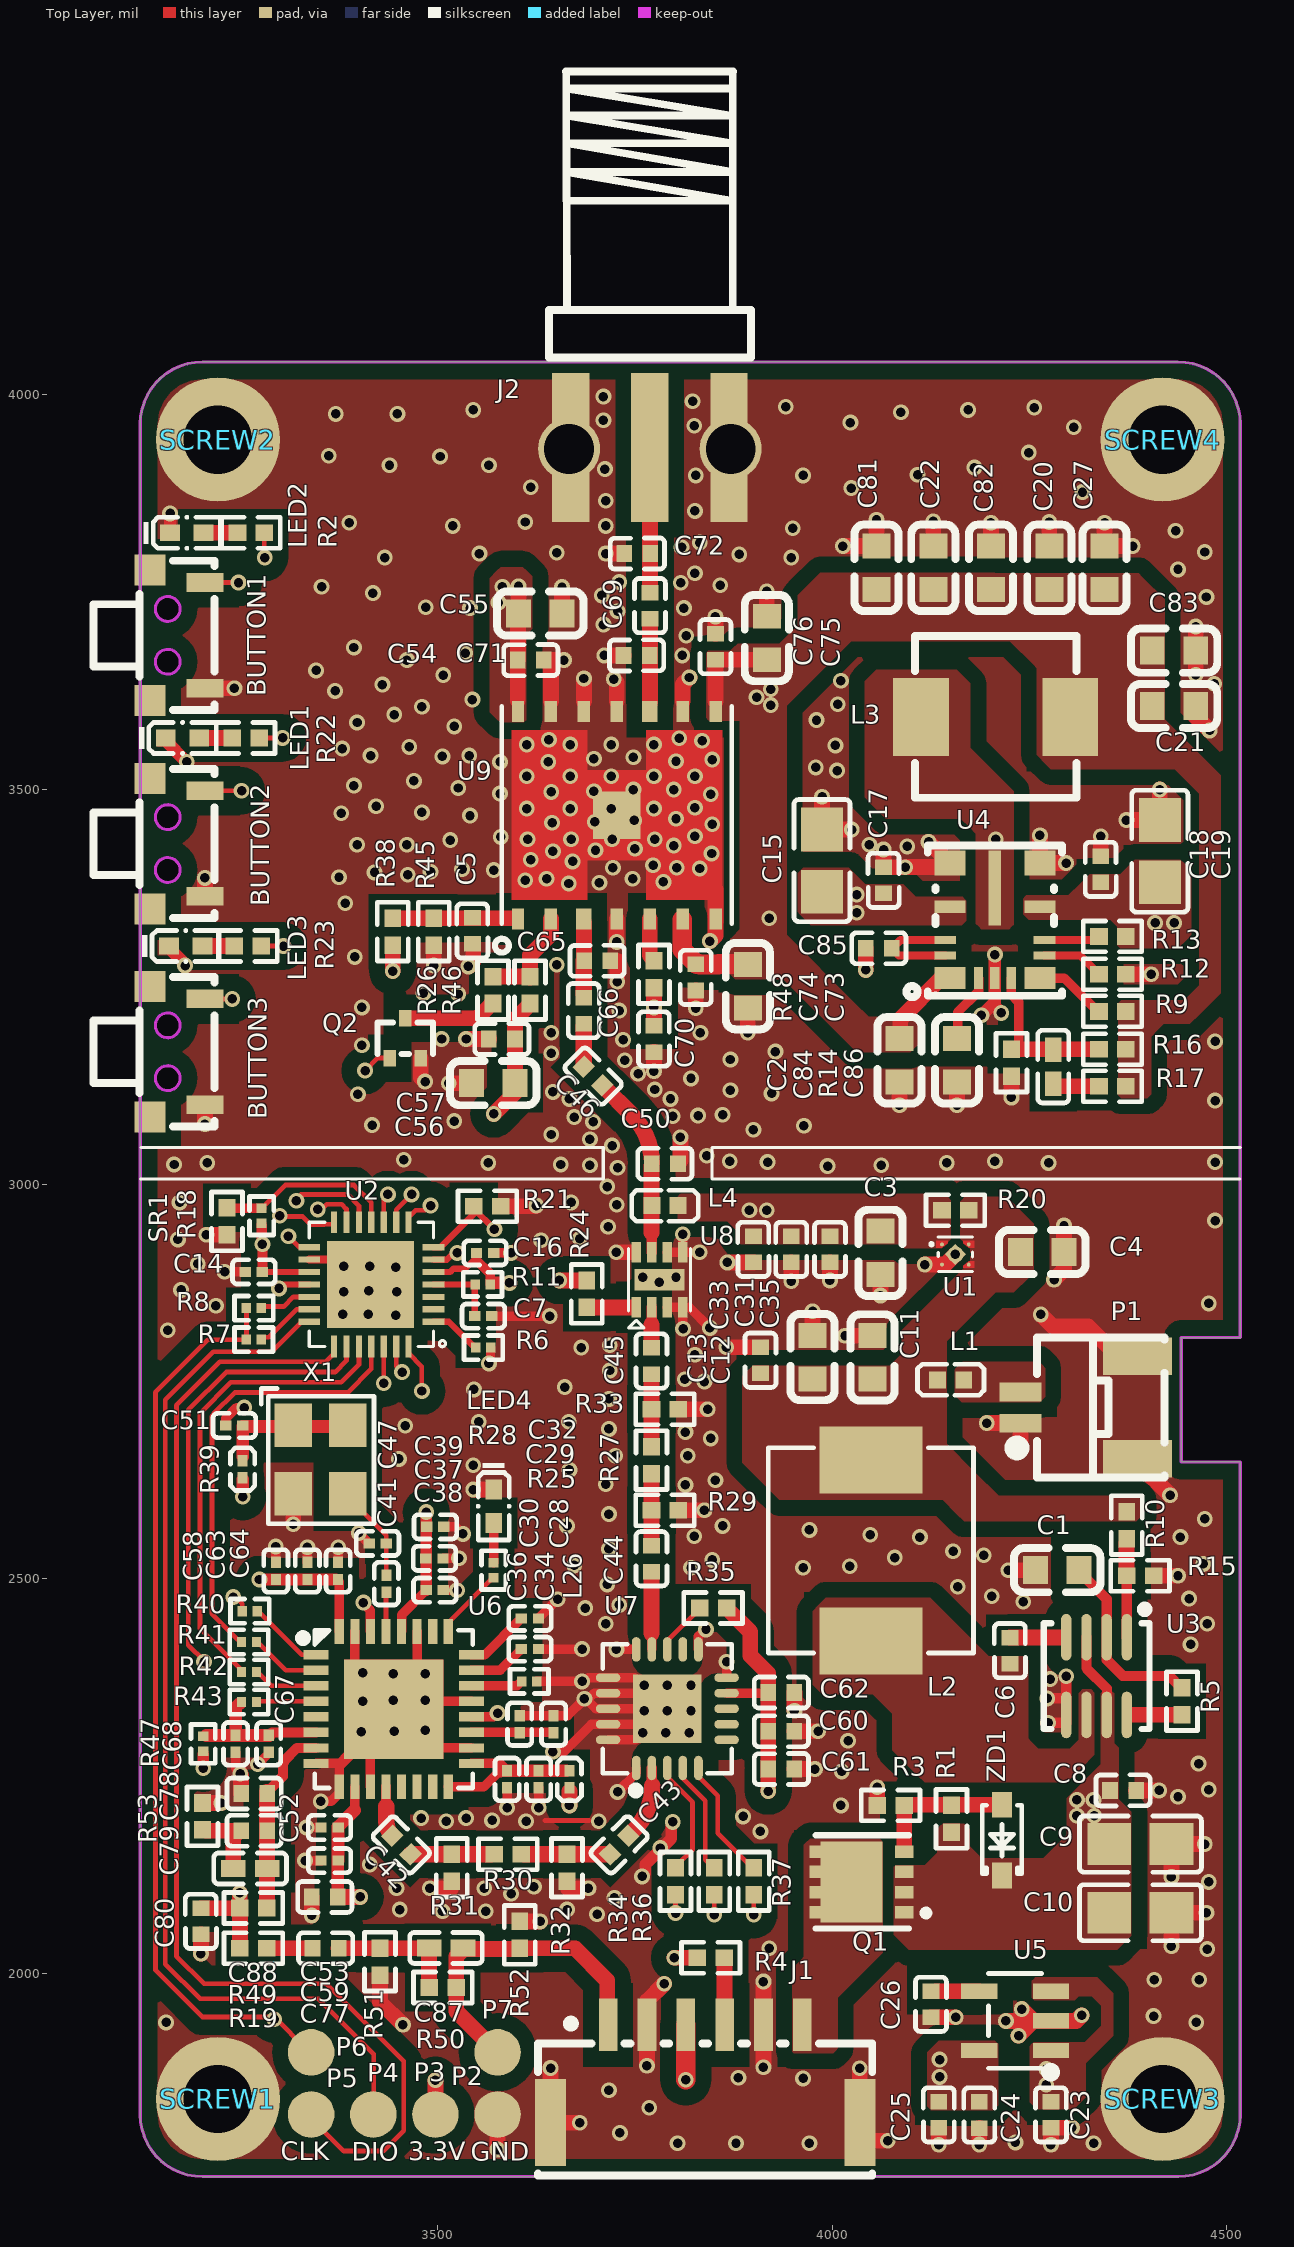
[diagram p0: Top Layer view]
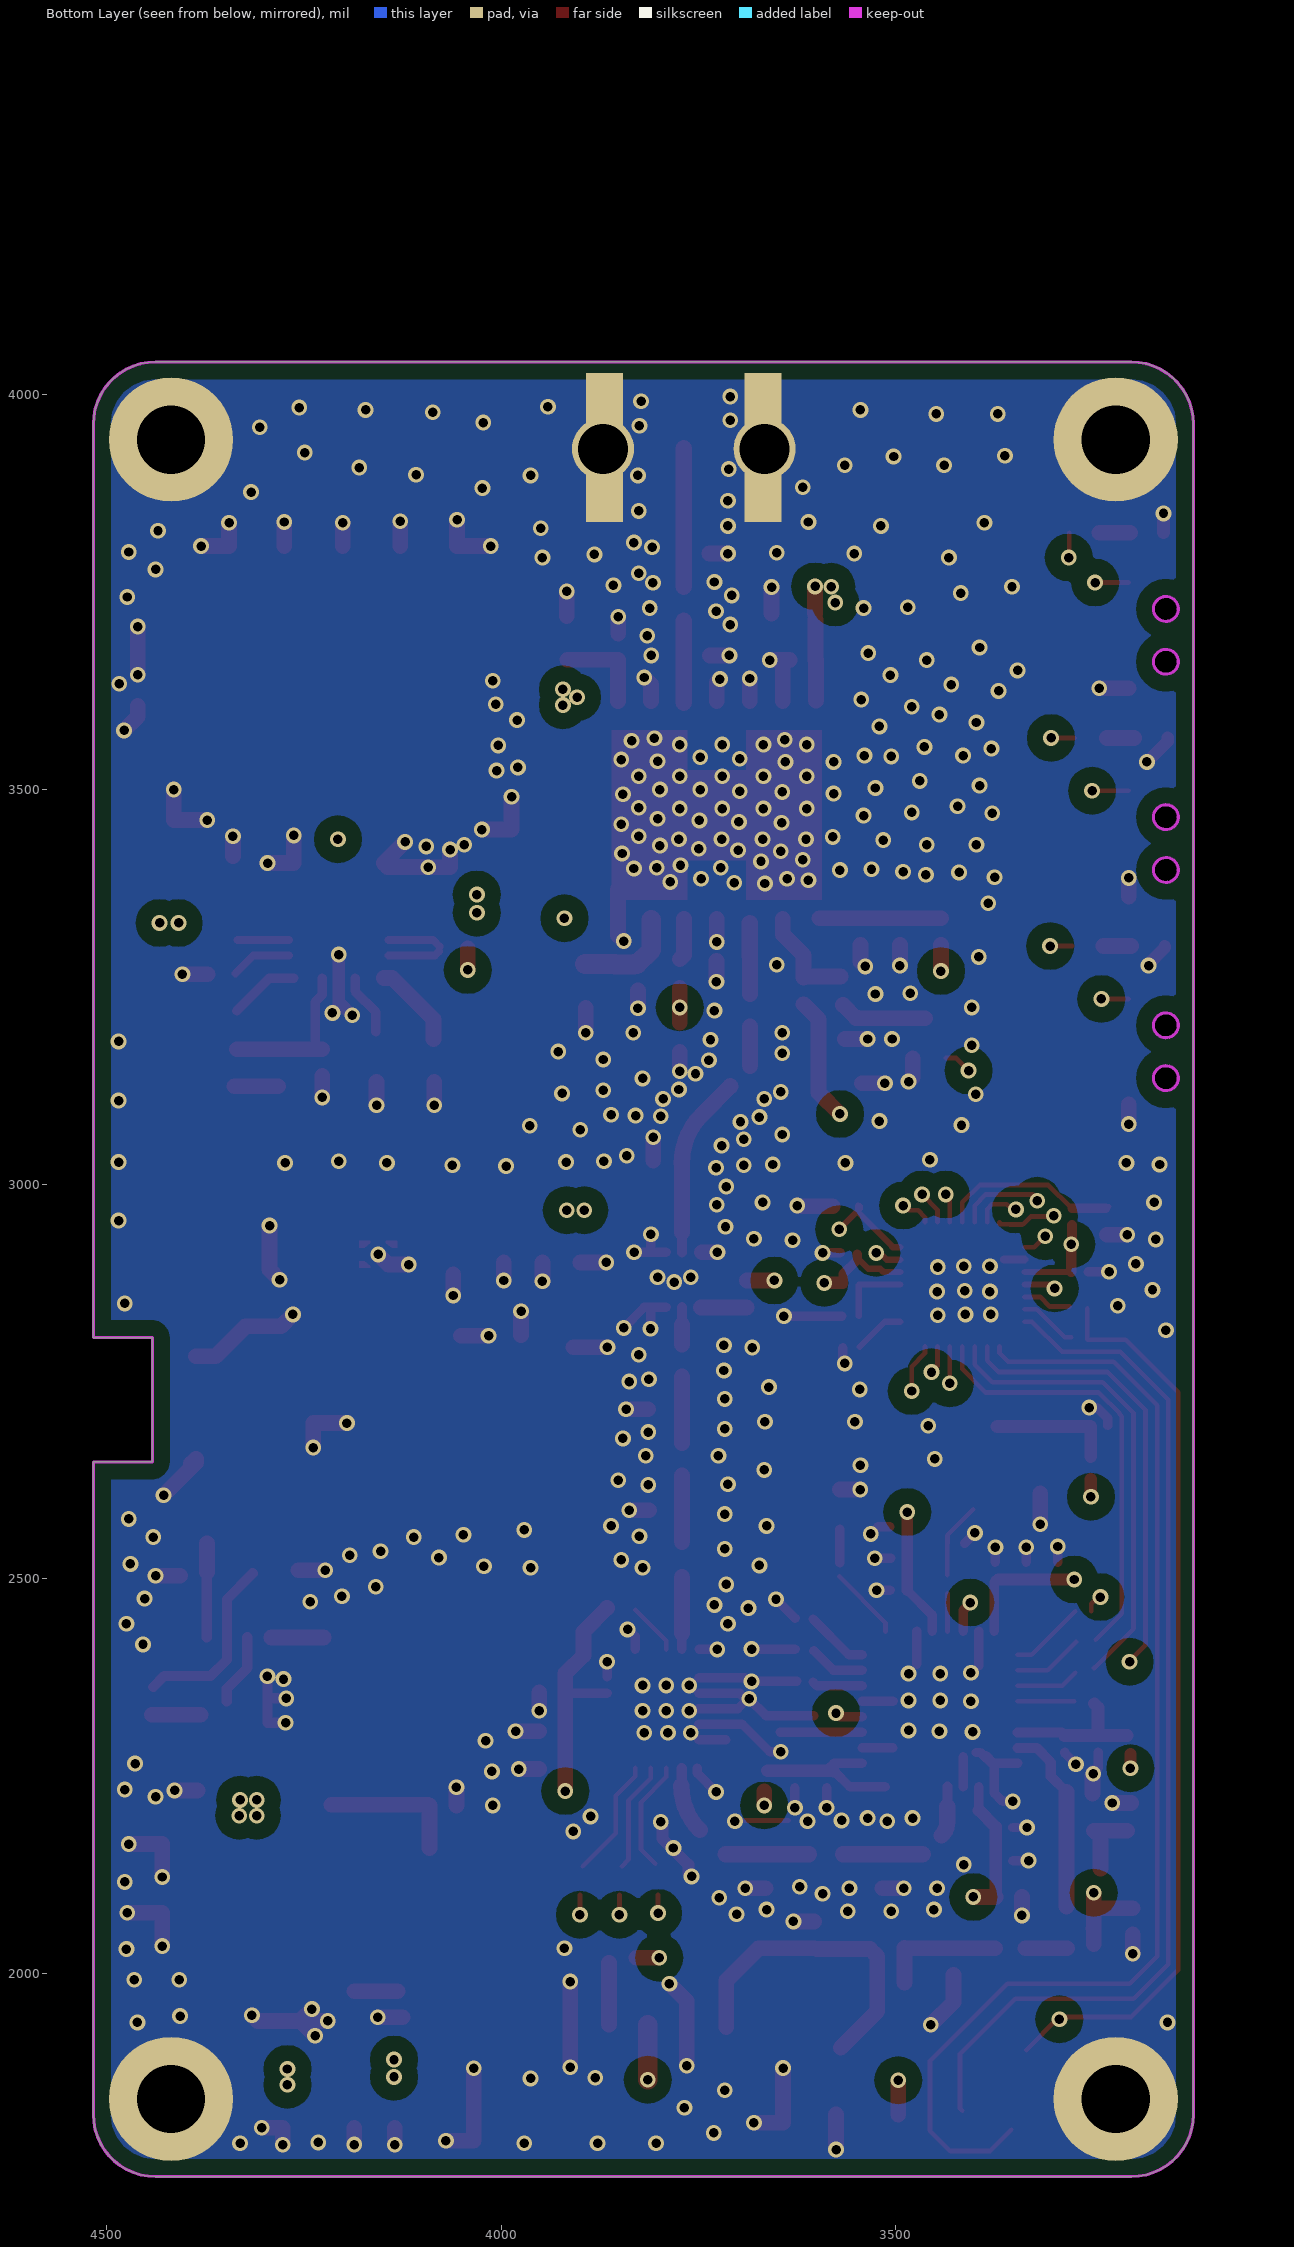
[diagram p1: Bottom Layer view, seen from below]
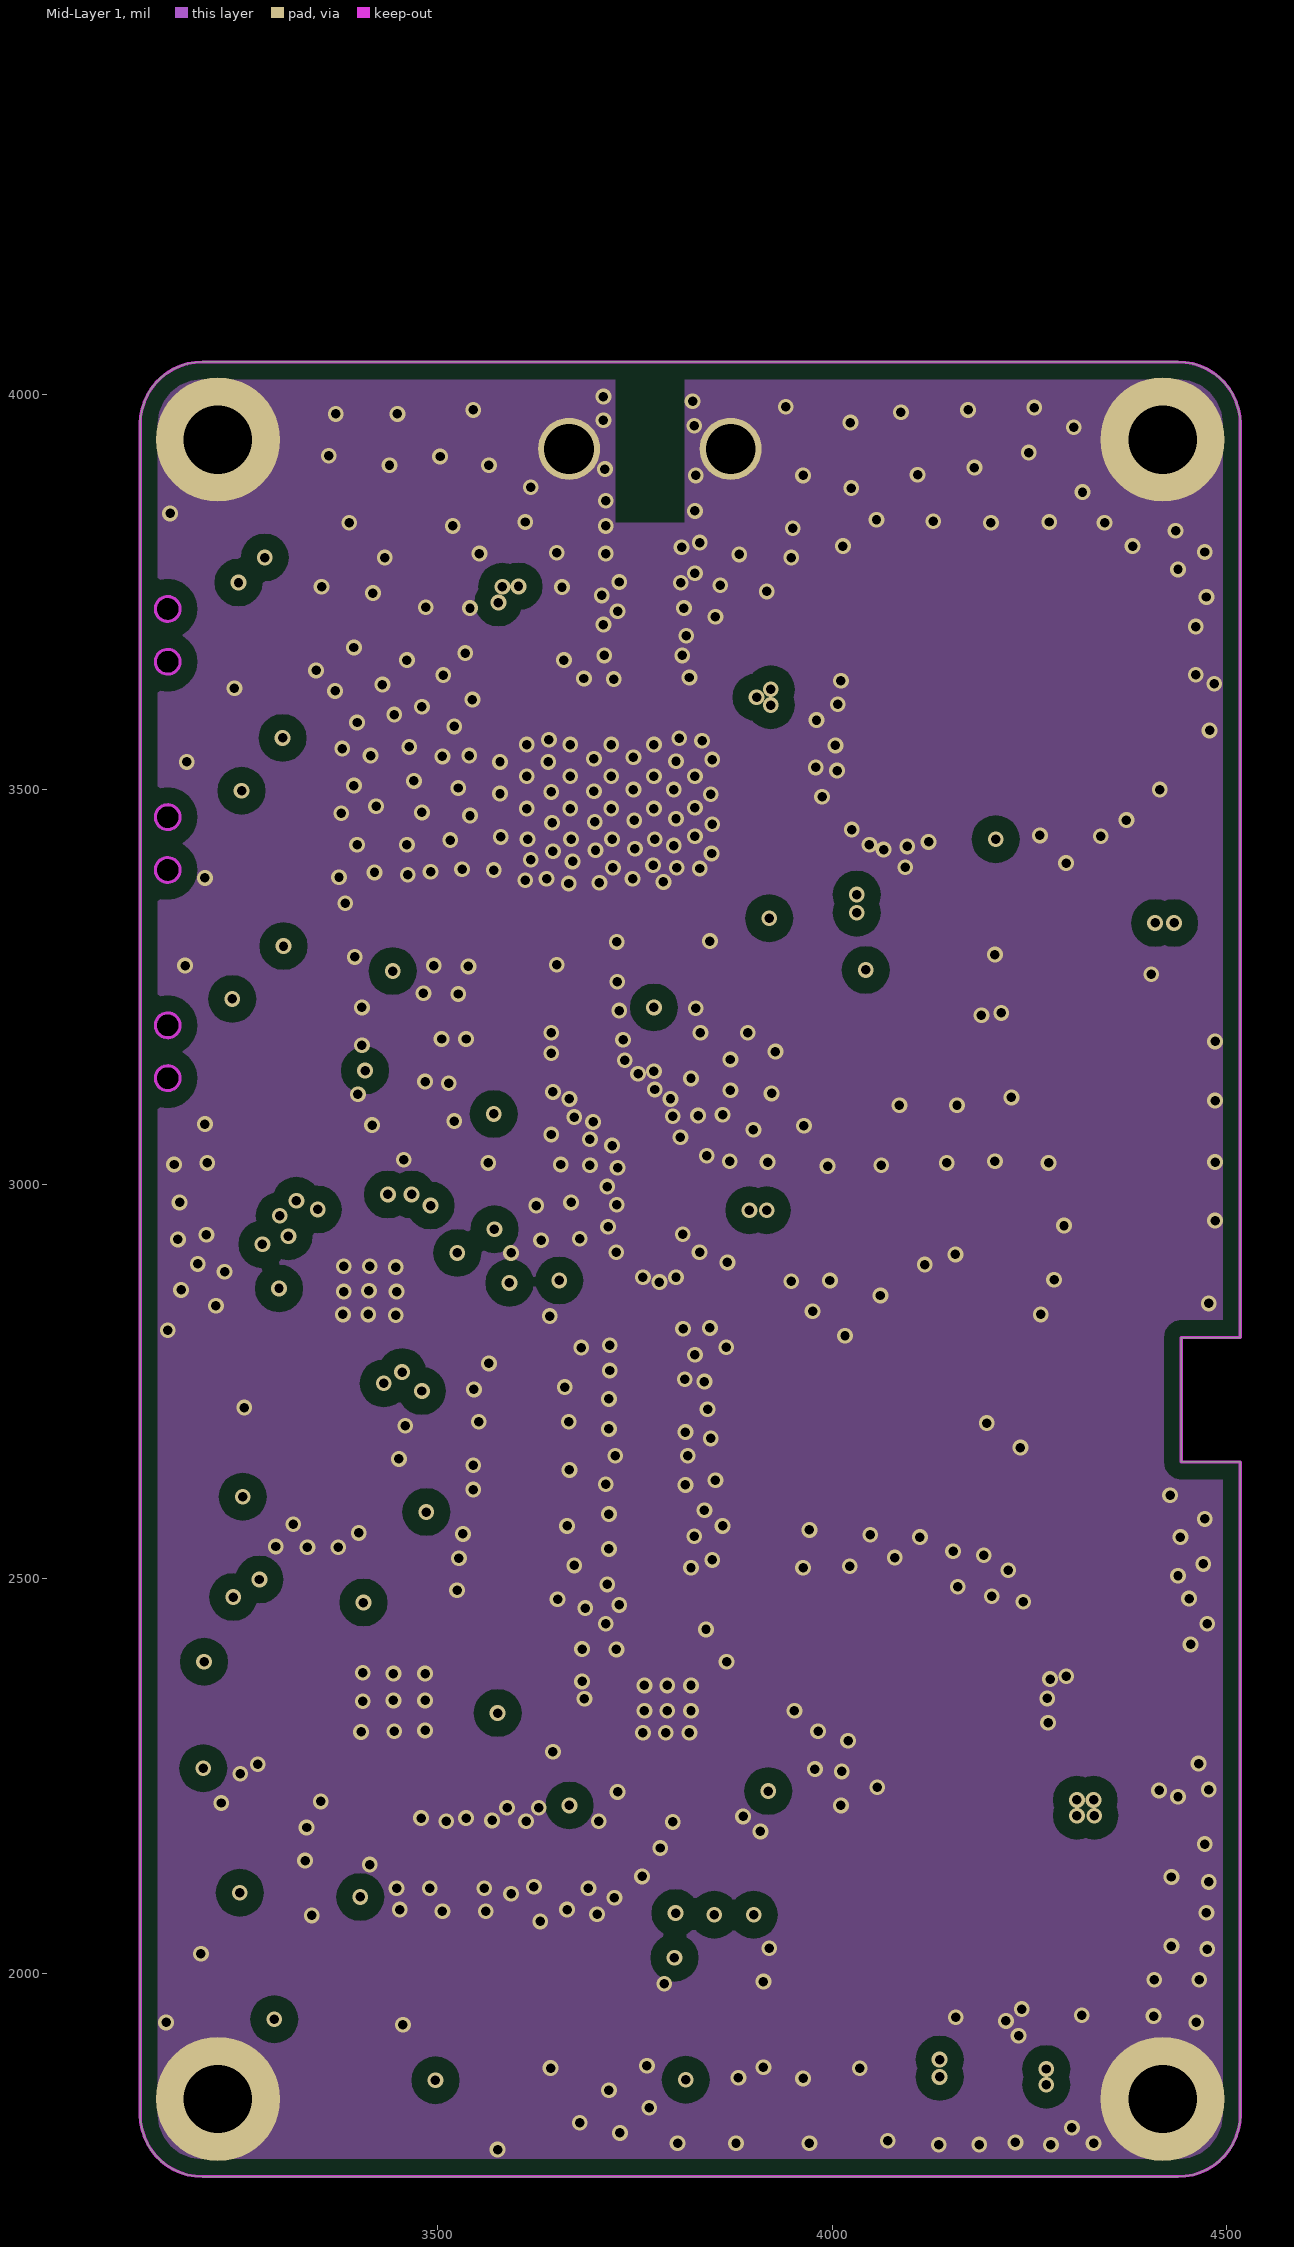
[diagram p2: Mid-Layer 1]
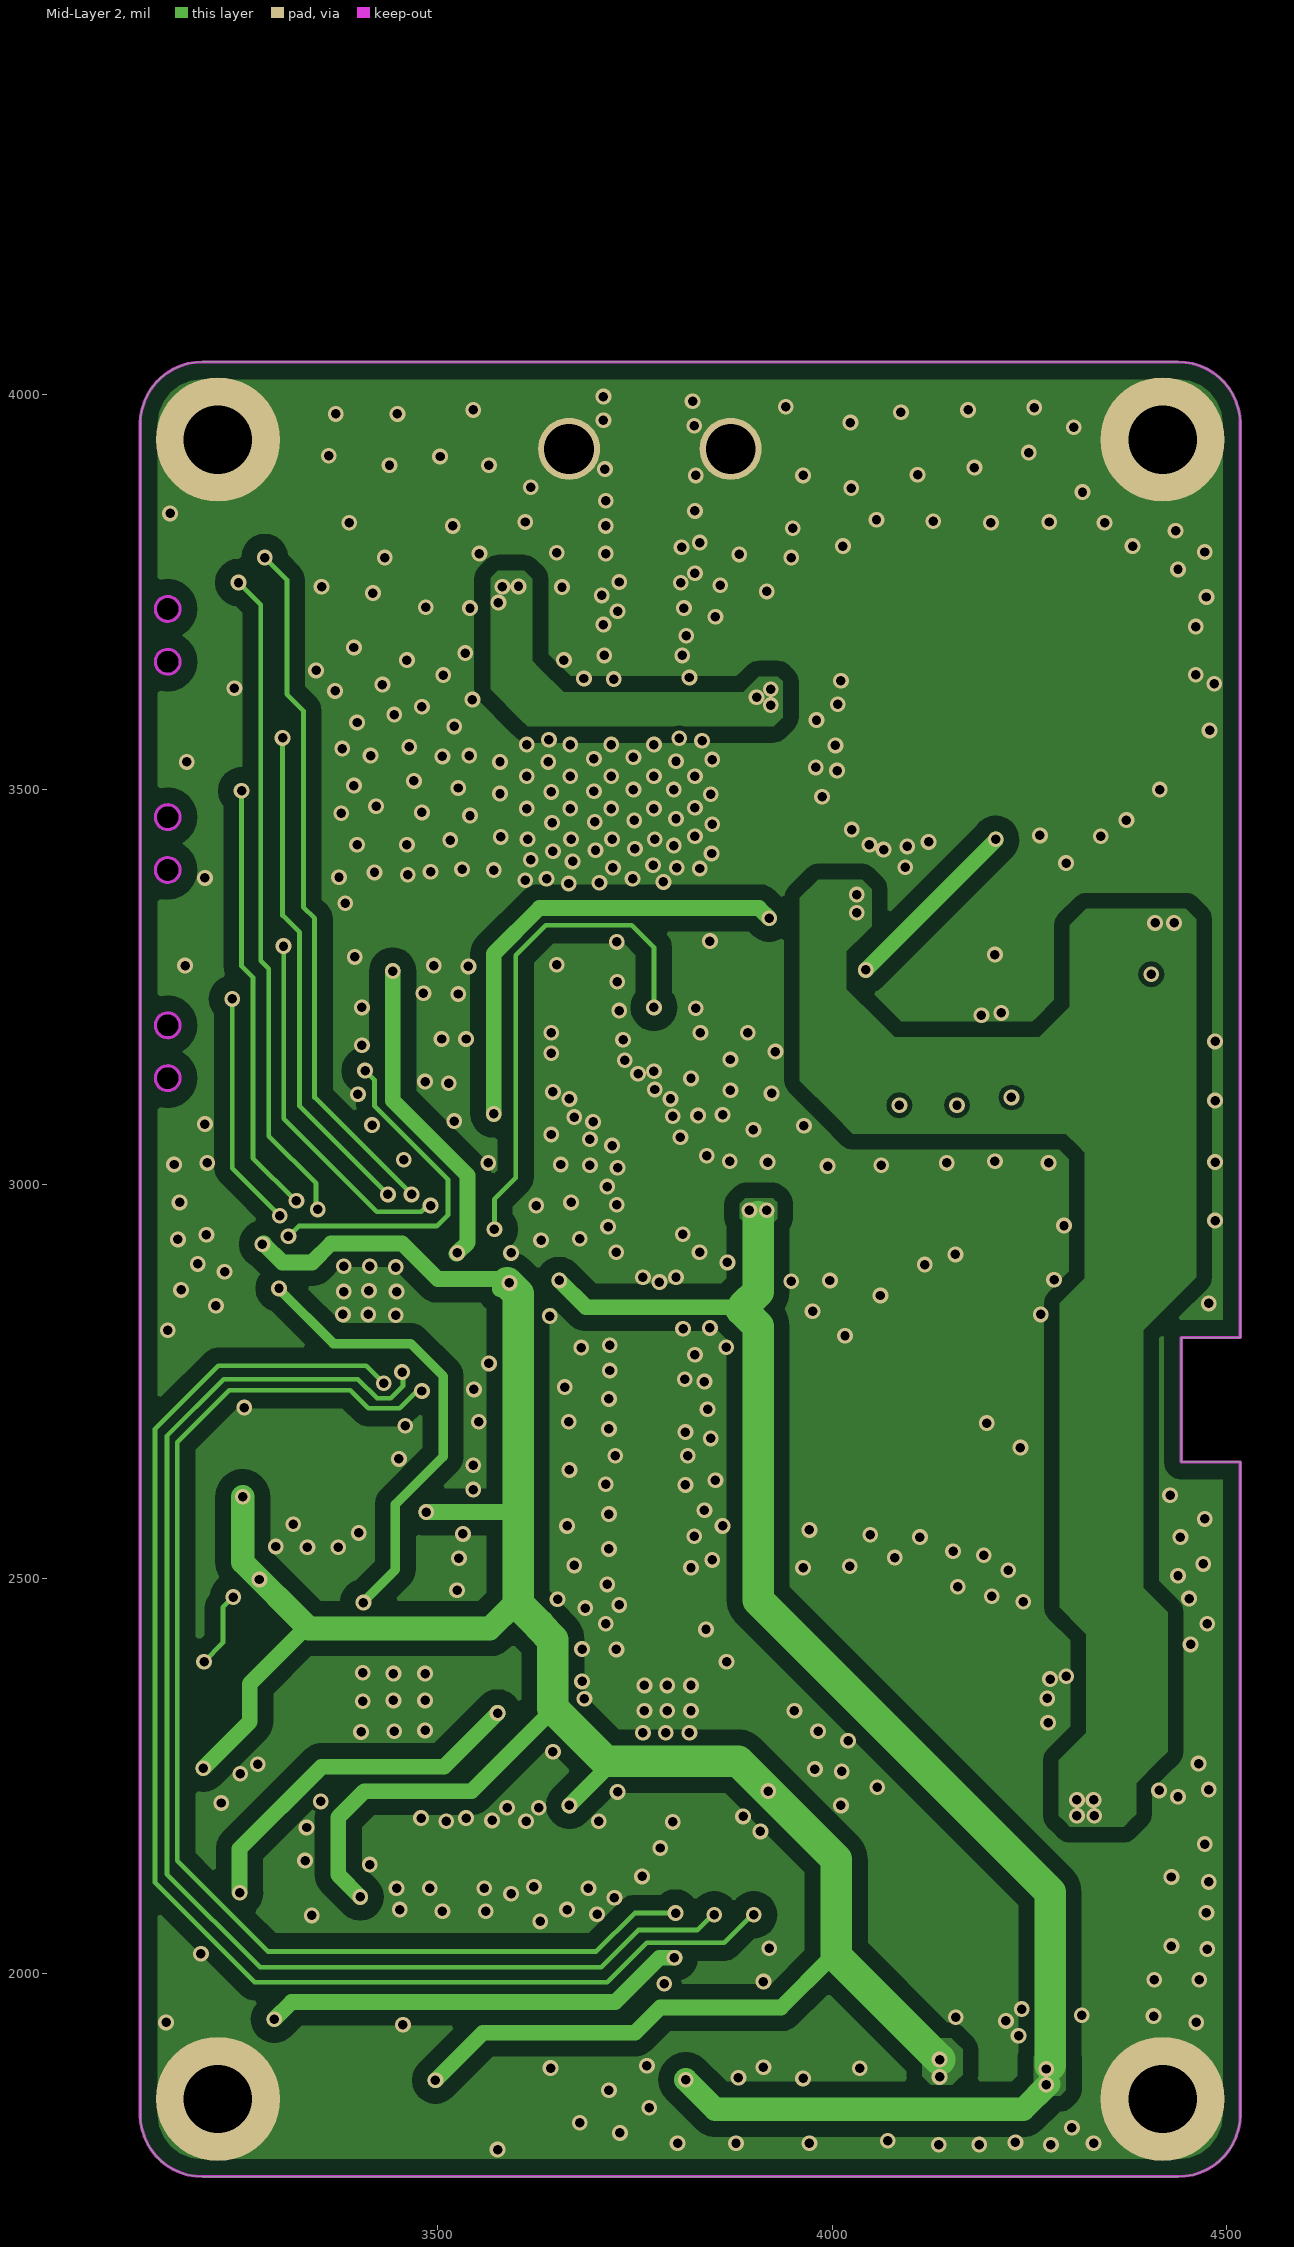
[diagram p3: Mid-Layer 2]
# Altium PCB MISC62792.PcbDoc (part 1 of 2)
Units mil, origin at the board's own origin, x right, y up, seen from the top; angles counter-clockwise.
Board outline 1393.7 x 2299.21 mil, 4 copper layers (Top Layer, Mid-Layer 1, Mid-Layer 2, Bottom Layer); 176 components, 94 nets, 498 pads, 570 vias.

## Layer stack, top to bottom (the 12.6 mil dielectric is the usual default, probably not edited)
Top Layer: signal copper 1.4
Dielectric: core 12.6, FR-4, Dk 4.8
Mid-Layer 1: signal copper 1.4
Dielectric: prepreg 12.6, FR-4, Dk 4.8
Mid-Layer 2: signal copper 1.4
Dielectric: core 12.6, FR-4, Dk 4.8
Bottom Layer: signal copper 1.4

## Board outline
3123.19,1821.38 ccw(c3201.93,1821.38) 3201.93,1742.64 4438.15,1742.64 ccw(c4438.15,1821.38) 4516.89,1821.38 4516.89,2648.15 4442.09,2648.15 4442.09,2805.63 4516.89,2805.63 4516.89,3963.11 ccw(c4438.15,3963.11) 4438.15,4041.85 3201.93,4041.85 ccw(c3201.93,3963.11) 3123.19,3963.11

## Design rules (kind name [scope] priority, off if disabled: settings)
Clearance Clearance_5 [INPOLYGON] p1: gap=6
Clearance [All] p2: gap=6
DiffPairsRouting [All] p1: maxlimit=6 minlimit=6 mostfreqgap=6 maxuncoupledlength=500
HoleSize [All] p1: absolutevalues=TRUE maxlimit=500 minlimit=1 maxpercent=80.000 minpercent=20.000
HoleToHoleClearance [All] p1: gap=0 allowstackedmicrovias=TRUE
MinimumSolderMaskSliver [All] p1: minsoldermaskwidth=0
PlaneClearance [All] p1: clearance=6
PlaneConnect [All] p1: planeconnectstyle=Direct reliefexpansion=20 reliefentries=4 reliefconductorwidth=10 reliefairgap=10
PolygonConnect [All] p1: connectstyle=Direct reliefconductorwidth=10 reliefentries=4 polygonreliefangle="90 Angle"
RoutingVias [All] p1: holewidth=12 width=20 viastyle="Through Hole" minholewidth=12 minwidth=20 maxholewidth=12 maxwidth=20
SilkToSilkClearance [All] p1: silktosilkclearance=0
SilkscreenOverComponentPads [All] p1: minsilkscreentomaskgap=0
SolderMaskExpansion [All] p1: expansion=4
Width [All] p1: maxlimit=100 minlimit=6 preferedwidth=6
20 further rules are at their usual default settings.

## Components (designator, comment, footprint, x,y, rotation, side; value= is the part's Value field where it differs from the comment)
BUTTON1 "TS24CA250GF013" SW-SMD_L4.7-W3.5-P3.35-EH 3170.43,3695.39 r0 top
BUTTON2 "TS24CA250GF013" SW-SMD_L4.7-W3.5-P3.35-EH 3170.43,3431.61 r0 top
BUTTON3 "TS24CA250GF013" SW-SMD_L4.7-W3.5-P3.35-EH 3170.43,3167.83 r0 top
C1 "1uf" C0603 4285,2511 r180 top
C2 "1uf" C0603 4085,3157 r270 top
C3 "1uF" C0603 4061,2913 r270 top
C4 "1uF" C0603 4266,2914 r0 top
C5 "0.1uF" C0402#1 3544,3321 r90 top
C6 "0.1uF" C0402#1 4225,2409 r270 top
C7 "100nf" C0201 3558,2833 r180 top
C8 "100nf" C0402#1 4368.37,2232 r0 top
C9 "10uF" C0805 4390.37,2164 r0 top
C10 "10uF" C0805 4390.37,2077 r0 top
C11 "22uF" C0603 4051,2780.56 r90 top
C12 "22uF" C0603 3975,2781 r90 top
C13 "100nf" C0402#1 3909,2777 r90 top
C14 "100nf" C0201 3267.2,2889 r180 top
C15 "10uF" C0805 3987,3410 r90 top
C16 "100nf" C0201 3560,2913 r0 top
C17 "100nf" C0402#1 4065,3385 r90 top
C18 "100nf" C0402#1 4340,3399 r90 top
C19 "10uF" C0805 4415,3422 r90 top
C20 "22uF" C0603 4275,3781 r90 top
C21 "22uF" C0603 4433,3606 r0 top
C22 "22uF" C0603 4128,3781 r90 top
C23 "1uF" C0402#1 4277,1821 r270 top
C24 "1uF" C0402#1 4186.33,1820.72 r270 top
C25 "100nf" C0402#1 4135,1821 r270 top
C26 "3.3nf" C0402#1 4125,1961 r270 top
C27 "22uF" C0603 4345,3781 r90 top
C28 "0.1uF" C0201 3647,2316 r270 top
C29 "0.1uF" C0201 3617,2411 r0 top
C30 "1NF" C0201 3604,2316 r90 top
C31 "1UF" C0402#1 3948,2917.46 r90 top
C32 "1NF" C0201 3617,2450 r180 top
C33 "100nf" C0402#1 3900,2917.46 r90 top
C34 "0.1uF" C0201 3628,2246 r90 top
C35 "10PF   50V" C0402#1 3997,2917.46 r270 top
C36 "1NF" C0201 3588,2246 r270 top
C37 "0.1uF" C0201 3496,2526 r180 top
C38 "1NF" C0201 3496.46,2485.62 r0 top
C39 "0.1uF" C0201 3497,2566 r180 top
C41 "1NF" C0201 3435,2494 r90 top
C42 "10PF" C0402#1 3454,2163 r315 top
C43 "10PF" C0402#1 3730,2163 r45 top
C44 "10PF" C0402#1 3771,2525.46 r90 top
C45 "10PF" C0402#1 3771,2776 r90 top
C46 "10PF" C0402#1 3697,3137 r135 top
C47 "1NF" C0201 3424,2545 r180 top
C50 "NC" C0402#1 3788,3026 r0 top
C51 "1NF" C0201 3242.35,2694.31 r0 top
C52 "100PF" C0201 3363,2185 r180 top
C53 "0.1uF" C0201 3363,2143 r0 top
C54 "10PF" C0402#1 3618,3664 r0 top
C55 "4.7UF" C0603 3630,3723 r0 top
C56 "4.7UF" C0603 3570.46,3128 r0 top
C57 "10PF" C0402#1 3581.46,3184 r0 top
C58 "1NF" C0201 3295,2510 r270 top
C59 "10uF" C0402#1 3357,2097 r0 top
C60 "1NF" C0402#1 3935.46,2307 r180 top
C61 "100nf" C0402#1 3935.46,2259 r180 top
C62 "1UF" C0402#1 3935.46,2356 r180 top
C63 "1NF" C0201 3335,2510 r270 top
C64 "1NF" C0201 3374,2510 r90 top
C65 "NC" C0402#1 3702,3283 r0 top
C66 "10PF" C0402#1 3685,3220 r270 top
C67 "1NF" C0201 3286,2291 r270 top
C68 "0.1uF" C0201 3244,2291 r90 top
C69 "10PF" C0402#1 3769,3733 r90 top
C70 "2.2NF" C0402#1 3774,3184 r90 top
C71 "NC" C0402#1 3752,3670 r0 top
C72 "NC" C0402#1 3753,3799 r0 top
C73 "4.7uF" C0603 3893,3251 r270 top
C74 "10PF" C0402#1 3827,3262 r270 top
C75 "4.7UF" C0603 3917,3692 r90 top
C76 "10PF" C0402#1 3852,3681 r90 top
C77 "4.7UF" C0402#1 3358,2032 r180 top
C78 "4.7UF" C0402#1 3267.42,2228 r180 top
C79 "22UF" C0402#1 3267.42,2181 r0 top
C80 "2PF" C0402#1 3200,2066 r90 top
C81 "22uF" C0603 4056,3781 r90 top
C82 "22uF" C0603 4201,3781 r90 top
C83 "1uf" C0603 4433,3676 r0 top
C84 "1uf" C0603 4158,3157 r270 top
C85 "0.1uF" C0402#1 4059,3299 r180 top
C86 "22pF" C0402#2 4280,3149 r270 top
C87 "150PF" C0402#2 3510.63,2032.41 r180 top
C88 "22UF" C0402#2 3262.42,2133 r0 top
J1 "WAFER-GH1. 25-6PWB" SMD_6P-P1.25_XUNPU_WAFER-GH1.25-6PWB 3838.98,1872.99 r0 top locked
J2 "SMA-50KE-3" SMA-FP-945G 3768.86,3931.61 r90 top locked
L1 "MPZ1005S121CT000" L0402 4150,2752 r180 top
L2 "SL0624-100M" IND-SMD_L7.1-W6.6 4049,2536 r90 top
L3 "MCS0530-4R7MN2" IND-SMD_L5.2-W5.2_YSPI0530 4207,3592 r0 top
L4 "33nH" L0402 3788,2973 r0 top
L26 "BLM03PX800SN1D" L0201 3667,2246 r90 top
LED1 "LED" LED0402 3176.8,3565.47 r0 top
LED2 "LED" LED0402 3182.24,3825.31 r0 top
LED3 "LED" LED0402 3180.74,3301.69 r0 top
LED4 "LED" LED0402 3571,2592 r270 top
P1 "WAFER-SHB1.0-2PWB" SMD_2P-WAFER-SHB1.0-2PWB 4312.66,2717.05 r90 top locked
P2 "Pad" PAD 3575.94,1821.38 r0 top locked
P3 "Pad" PAD 3497.2,1821.38 r0 top locked
P4 "Pad" PAD 3418.46,1821.38 r0 top locked
P5 "Pad" PAD 3339.72,1821.38 r0 top locked
P6 "Pad" PAD 3339.72,1900.12 r0 top
P7 "Pad" PAD 3575.94,1900.12 r0 top locked
Q1 "CJAE10P06" DFN-8_L3.0-W3.0-P0.65-BL_G48N03D3 4037,2116 r90 top
Q2 "DULCTU3134K" SOT-523-3_L1.6-W0.8-P0.50-LS1.6-BR-1 3459,3185 r270 top
R1 "50K" R0402 4151,2196 r270 top
R2 "3.3K" R0402 3263.43,3825.31 r180 top
R3 "100K" R0402 4074,2213 r0 top
R4 "1K" R0402 3846,2020 r180 top
R5 "100K" R0402 4443,2345 r270 top
R6 "10K" R0201 3558,2793 r180 top
R7 "22R" R0201 3267,2803 r180 top
R8 "22R" R0201 3267.2,2843 r180 top
R9 "100K" R0402 4355,3219 r0 top
R10 "107K" R0402 4373,2568 r270 top
R11 "10K" R0201 3557,2873 r0 top
R12 "33.2K" R0402 4355,3266 r0 top
R13 "10K" R0402 4355,3314 r0 top
R14 "24.9K" R0402 4227,3154 r270 top
R15 "24.9K" R0402 4390,2504 r0 top
R16 "113K" R0402 4355,3171 r180 top
R17 "1K" R0402 4355,3124 r180 top
R18 "10K" R0201 3277,2960 r90 top
R19 "2K" R0402 3266.42,2032 r0 top
R20 "NC" R0402 4156,2967 r0 top
R21 "10K" R0402 3563,2972 r0 top
R22 "3.3K" R0402 3256.8,3565.47 r180 top
R23 "3.3K" R0402 3259.55,3301.69 r180 top
R24 "3.9K" R0402 3689,2861 r270 top
R25 "4.7K" R0201 3616,2370 r180 top
R26 "1K" R0402 3570,3246 r270 top
R27 "30R" R0402 3771,2650.46 r90 top
R28 "4.7K" R0201 3571,2511 r270 top
R29 "180R" R0402 3788,2587 r0 top
R30 "18R" R0402 3588.92,2151 r0 top
R31 "300R" R0402 3518,2134 r270 top
R32 "300R" R0402 3664,2134 r270 top
R33 "180R" R0402 3788,2715 r0 top
R34 "0R" R0402 3801.37,2116.91 r270 top
R35 "0R" R0402 3849,2463 r0 top
R36 "0R" R0402 3850.37,2116.91 r270 top
R37 "0R" R0402 3900.37,2116.91 r270 top
R38 "0R" R0402 3443,3320 r90 top
R39 "BLM03PX800SN1D" L0201 3253,2639 r90 top
R40 "0R" R0201 3262,2459 r180 top
R41 "0R" R0201 3261,2420 r180 top
R42 "0R" R0201 3261,2382 r180 top
R43 "0R" R0201 3261,2344 r180 top
R45 "1MR" R0402 3495,3320 r270 top
R46 "1K" R0402 3617,3246 r90 top
R47 "0R" R0201 3203,2291 r270 top
R48 "" R0402 3774,3266 r90 top
R49 "20K" R0402 3266.42,2083 r180 top
R50 "270R" R0402 3506.63,1982.41 r0 top
R51 "10R" R0402 3427,2015 r270 top
R52 "91R" R0402 3604,2049 r90 top
R53 "22R" R0402 3202,2199 r90 top
SCREW1 "MARK_4" M2 3221.61,1841.06 r90 top locked
SCREW2 "MARK_4" M2 3221.61,3943.43 r90 top locked
SCREW3 "MARK_4" M2 4418.46,1841.06 r90 top locked
SCREW4 "MARK_4" M2 4418.46,3943.43 r90 top locked
SR1 "SDNT1005X103F3380FTF" R0402 3233,2953 r270 top
U1 "TPS7A2050PDQNR" X2SON-4_L1.0-W1.0-P0.65-TL-EP 4156,2910.99 r0 top
U2 "GD32E230G8U6" QFN-28_L4.0-W4.0-P0.40-BL-EP2.8 3416,2873 r90 top
U3 "AWK6943" QFN-8_L3.0-W3.0-P0.65-BL 4334.8,2376.79 r180 top
U4 "LM61460AASQRJRRQ1" VQFN-14-HR_L4.0-W3.5-TL_LM61460AASQRJRRQ1 4206,3334 r90 top
U5 "RT9013-33GB" SOT-23-5_L3.0-W1.7-P0.95-LS2.8-BL 4231.51,1940 r90 top
U6 "GX1288FL" QFN-32_L5.0-W5.0-P0.50 3444.42,2335 r0 top
U7 "ARW621A" QFN-20_L4.0-W4.0-P0.50-TL-EP2.2 3791,2335.46 r90 top
U8 "CBG9092" CBG9092 3781,2879 r90 top
U9 "32A" AU64XX 3727,3467.6 r90 top
X1 "OT322525MJBA4SL" SMD3225 3351.55,2651.31 r270 top
ZD1 "BZT52C15S" SOD-323_L1.7-W1.3-LS2.6-RD 4215,2169 r90 top

## Footprints (in the part's own frame and the unit in brackets; to place one, negate y for a bottom-side part, rotate by r counter-clockwise, add the part's x,y. Pads: shape width x height; smd on the part's side, far side on the other; paste and mask are expansions set on the pad)
AU64XX [mm]
  rect 0.675x0.4 smd paste+0 mask+0.05: 1(-3.337,3.18) 2(-3.337,2.12) 4(-3.337,0) 5(-3.337,-1.06) 6(-3.337,-2.12) 7(-3.337,-3.18) 8(3.338,-3.18) 9(3.338,-2.12) 11(3.338,0) 12(3.338,1.06) 13(3.338,2.12) 14(3.338,3.18)
  rect 0.675x0.5 smd paste+0 mask+0.05: 3(-3.337,1.06) 10(3.338,-1.06)
  rect 1.524x1.524 smd paste+0 mask+0.05: 15(0,0)
  Top Layer region: -2.725,-3.385 -2.725,-0.945 -1.45,-0.945 -1.45,0.945 -2.725,0.945 -2.725,3.385 2.725,3.385 2.725,0.945 1.45,0.945 1.45,-0.945 2.725,-0.945 2.725,-3.385
  silkscreen extent -4.42,-3.7 3.5,3.92
C0201 [mil]
  rect 14.51x12.76 smd paste-3937.01 mask+2: 1(-10.8,0) 2(10.8,0)
  silkscreen extent -27,-15 27,15
C0402#1 [mm]
  rect 0.5x0.54 smd paste+0.051: 1(-0.42,0) 2(0.42,0)
  silkscreen extent -0.87,-0.5 0.87,0.5
C0402#2 [mm]
  rect 0.79x0.54 smd paste-100 mask+0.051: 1(-0.545,0) 2(0.545,0)
  silkscreen extent -1.17,-0.5 1.17,0.5
C0603 [mm]
  rect 0.8x0.9 smd: 1(-0.7,0) 2(0.7,0)
  silkscreen extent -1.39,-0.71 1.39,0.71
C0805 [mm]
  rect 1.41x1.35 smd paste-100 mask+0.051: 1(-1,0) 2(1,0)
  silkscreen extent -1.96,-0.9 1.96,0.9
CBG9092 [mm]
  rect 0.67x0.3 smd: 1(-0.885,0.75) 2(-0.885,0.25) 3(-0.885,-0.25) 4(-0.885,-0.75) 5(0.885,-0.75) 6(0.885,-0.25) 7(0.885,0.25) 8(0.885,0.75)
  rect 0.7x1.6 smd: 9(0,0)
  silkscreen extent -1.55,-1 1,1
DFN-8_L3.0-W3.0-P0.65-BL_G48N03D3 [mm]
  rect 0.4x0.6 smd paste-100 mask+0.051: 1(-0.975,-1.375) 2(-0.325,-1.375) 3(0.325,-1.375) 4(0.975,-1.375) 5(0.975,1.375) 6(0.325,1.375) 7(-0.325,1.375) 8(-0.975,1.375)
  rect 2.6x2 smd paste-100 mask+0.051: 9(0,0.325)
  silkscreen extent -1.5,-2.18 1.5,1.48
IND-SMD_L5.2-W5.2_YSPI0530 [mm]
  rect 1.8x2.5 smd: 1(-2.4,0) 2(2.4,0)
  silkscreen extent -2.6,-2.6 2.6,2.6
IND-SMD_L7.1-W6.6 [mm]
  rect 2.15x3.32 smd: 1(-2.913,0) 2(2.913,0)
  silkscreen extent -3.3,-3.3 3.3,3.3
L0201 [mil]
  rect 14.51x12.76 smd paste-3937.01 mask+2: 1(-10.8,0) 2(10.8,0)
  silkscreen extent -27,-15 27,15
L0402 [mm]
  rect 0.54x0.54 smd paste+0.051: 1(-0.42,0) 2(0.42,0)
  silkscreen extent -1.07,-0.51 1.07,0.49
LED0402 [mm]
  rect 0.636x0.54 smd paste-100 mask+0.051: 1(0.538,0) 2(-0.538,0)
  silkscreen extent -1.39,-0.54 1.09,0.54
M2 [mm]
  round 4 hole 2.2: 1(0,0)
PAD [mm]
  round 1.5 smd: 1(0,0)
QFN-8_L3.0-W3.0-P0.65-BL [mm]
  oval 0.33x1.5 smd: 1(-0.975,-1.25) 2(-0.325,-1.25) 3(0.325,-1.25) 4(0.975,-1.25) 5(0.975,1.25) 6(0.325,1.25) 7(-0.325,1.25) 8(-0.975,1.25)
  silkscreen extent -1.7,-2.27 1.7,1.7
QFN-20_L4.0-W4.0-P0.50-TL-EP2.2 [mm]
  oval 0.79x0.28 smd paste-100 mask+0.05: 1(-1.908,1) 2(-1.908,0.5) 3(-1.908,0) 4(-1.908,-0.5) 5(-1.908,-1) 11(1.908,-1) 12(1.908,-0.5) 13(1.908,0) 14(1.908,0.5) 15(1.908,1)
  oval 0.28x0.79 smd paste-100 mask+0.05: 6(-1,-1.908) 7(-0.5,-1.908) 8(0,-1.908) 9(0.5,-1.908) 10(1,-1.908) 16(1,1.908) 17(0.5,1.908) 18(0,1.908) 19(-0.5,1.908) 20(-1,1.908)
  rect 2.2x2.2 smd paste-100 mask+0.05: 21(0,0)
  silkscreen extent -2.76,-2.08 2.08,2.08
QFN-28_L4.0-W4.0-P0.40-BL-EP2.8 [mm]
  rect 0.2x0.7 smd paste-100 mask+0.051: 1(-1.2,-2) 2(-0.8,-2) 3(-0.4,-2) 4(-0.001,-2) 5(0.4,-2) 6(0.8,-2) 7(1.2,-2) 15(1.2,2) 16(0.8,2) 17(0.4,2) 18(0,2) 19(-0.4,2) 20(-0.8,2) 21(-1.2,2)
  rect 0.7x0.2 smd paste-100 mask+0.051: 8(2,-1.2) 9(2,-0.8) 10(2,-0.4) 11(1.999,0) 12(2,0.4) 13(2,0.8) 14(2,1.2) 22(-2,1.2) 23(-2,0.8) 24(-2,0.4) 25(-2,0) 26(-2,-0.4) 27(-2,-0.8) 28(-2,-1.2)
  rect 2.8x2.8 smd paste-100 mask+0.051: 29(0,0.02)
  silkscreen extent -2,-2.39 2,2
QFN-32_L5.0-W5.0-P0.50 [mm]
  rect 0.8x0.3 smd paste-100 mask+0.051: 1(-2.5,1.75) 2(-2.5,1.25) 3(-2.5,0.75) 4(-2.5,0.25) 5(-2.5,-0.25) 6(-2.5,-0.75) 7(-2.5,-1.25) 8(-2.5,-1.75) 17(2.5,-1.75) 18(2.5,-1.25) 19(2.5,-0.75) 20(2.5,-0.25) 21(2.5,0.25) 22(2.5,0.75) 23(2.5,1.25) 24(2.5,1.75)
  rect 0.3x0.8 smd paste-100 mask+0.051: 9(-1.75,-2.5) 10(-1.25,-2.5) 11(-0.75,-2.5) 12(-0.25,-2.5) 13(0.25,-2.5) 14(0.75,-2.5) 15(1.25,-2.5) 16(1.75,-2.5) 25(1.75,2.5) 26(1.25,2.5) 27(0.75,2.5) 28(0.25,2.5) 29(-0.25,2.5) 30(-0.75,2.5) 31(-1.25,2.5) 32(-1.75,2.5)
  rect 3.2x3.2 smd paste-100 mask+0.051: 33(0,0)
  silkscreen extent -3.05,-2.54 2.54,2.54
R0201 [mil]
  rect 11.93x12.76 smd paste-3937.01 mask+2: 1(-9.51,0) 2(9.51,0)
  silkscreen extent -24,-15 24,15
R0402 [mm]
  rect 0.566x0.54 smd paste-100 mask+0.051: 1(-0.433,0) 2(0.433,0)
  silkscreen extent -0.94,-0.5 0.94,0.5
SMA-FP-945G [mm] "SMA-FP-945G,侧装,卡板插孔"
  rect 4.8x1.2 smd: 1(0.05,0) 2(0.05,2.55) 2(0.05,-2.55)
  round 2 hole 1.6: 2(0,2.6) 2(0,-2.6)
  rect 4.8x1.2 smd far side: 2(0.05,2.55) 2(0.05,-2.55)
  silkscreen extent 2.94,-3.25 12.15,3.25
SMD3225 [mm]
  rect 1.4x1.2 smd paste+0.051: 1(-1.1,-0.875) 2(1.1,-0.875) 3(1.1,0.875) 4(-1.1,0.875)
  silkscreen extent -2.29,-1.9 2.07,1.72
SMD_2P-WAFER-SHB1.0-2PWB [mm]
  rect 0.6x1.35 smd paste+0 mask+0.05: 1(-0.5,1.887) 2(0.5,1.887)
  rect 1.2x2.22 smd paste+0 mask+0.05: 3(1.65,-1.887) 4(-1.65,-1.887)
  silkscreen extent -2.25,-2.75 2.25,2.2
SMD_6P-P1.25_XUNPU_WAFER-GH1.25-6PWB [mm]
  rect 0.6x1.7 smd paste+0 mask+0.05: 1(-3.125,1.575) 2(-1.875,1.575) 3(-0.625,1.575) 4(0.625,1.575) 5(1.875,1.575) 6(3.125,1.575)
  rect 1x2.8 smd paste+0 mask+0.05: 7(4.975,-1.575) 8(-4.975,-1.575)
  silkscreen extent -5.38,-3.27 5.37,1.74
SOD-323_L1.7-W1.3-LS2.6-RD [mm]
  rect 0.83x0.63 smd paste+0 mask+0.05: 1(1.14,0) 2(-1.14,0)
  silkscreen extent -1.08,-0.64 1.13,0.64
SOT-23-5_L3.0-W1.7-P0.95-LS2.8-BL [mm]
  rect 0.49x1.157 smd paste+0.051: 1(-0.95,-1.154) 2(0,-1.154) 3(0.95,-1.154)
  rect 0.49x1.175 smd paste+0.051: 4(0.95,1.154) 5(-0.95,1.154)
  silkscreen extent -1.8,-1.29 1.53,0.85
SOT-523-3_L1.6-W0.8-P0.50-LS1.6-BR-1 [mil]
  rect 21x16 smd paste+0 mask+1.97: 1(25.39,-19.68) 2(25.39,19.69)
  rect 21x15.75 smd paste+0 mask+1.97: 3(-25.4,0)
  silkscreen extent -20,-35 20,35
SW-SMD_L4.7-W3.5-P3.35-EH [mm]
  round 0.8 hole 0.8 unplated: 0(-0.315,-0.85) 0(-0.315,0.85)
  rect 1.2x0.6 smd paste+0 mask+0.05: 1(0.882,-1.7) 2(0.882,1.7)
  rect 1x1 smd paste+0 mask+0.05: 3(-0.882,2.1) 4(-0.882,-2.1)
  Keep-Out Layer circle w0.1: c-0.315,0.85 r0.4
  Keep-Out Layer circle w0.1: c-0.315,-0.85 r0.4
  silkscreen extent -2.71,-2.4 1.18,2.4
VQFN-14-HR_L4.0-W3.5-TL_LM61460AASQRJRRQ1 [mm]
  rect 0.7x1 smd paste+0 mask+0.05: 1(-1.85,1.45) 5(-1.85,-1.45)
  rect 0.7x0.3 smd paste+0 mask+0.05: 2(-1.85,0.525) 3(-1.85,0) 4(-1.85,-0.525)
  rect 0.25x0.7 smd paste+0 mask+0.05: 6(-1.125,-1.6) 7(-0.625,-1.6) 13(-0.625,1.6) 14(-1.125,1.6)
  rect 0.4x1 smd paste+0 mask+0.05: 8(0.45,-1.45) 12(0.45,1.45)
  rect 0.8x1 smd paste+0 mask+0.05: 9(1.85,-1.45) 11(1.85,1.45)
  rect 2.4x0.4 smd paste+0 mask+0.05: 10(1.05,0)
  silkscreen extent -2.47,-2.16 2.41,2.85
X2SON-4_L1.0-W1.0-P0.65-TL-EP [mm]
  round 0.125 smd: 1(-0.43,0.325) 2(-0.43,-0.325) 3(0.43,-0.325) 4(0.43,0.325)
  rect 0.48x0.48 smd rot 45 paste+0 mask+0.05: 5(0,0)
  Top Layer region: 0.61,0.435 0.61,0.215 0.43,0.215 0.25,0.355 0.25,0.435
  Top Layer region: -0.61,0.435 -0.61,0.215 -0.43,0.215 -0.25,0.355 -0.25,0.435
  Top Layer region: -0.61,-0.435 -0.61,-0.215 -0.43,-0.215 -0.25,-0.355 -0.25,-0.435
  Top Layer region: 0.61,-0.435 0.61,-0.215 0.43,-0.215 0.25,-0.355 0.25,-0.435
  silkscreen extent -0.82,-0.55 0.55,0.56

## Part data
BUTTON1 BUTTON2 BUTTON3: library part "TSW 3x6", "3x6 tactile switch"
C1 C2 C3 C4 C5 C6 C9 C10 C11 C12 C15 C19 C20 C21 C22 C23 C24 C26 C27 C28 C29 C30 C31 C32 C34 C35 C36 C37 C38 C39 C41 C42 C43 C44 C45 C46 C47 C50 C51 C52 C53 C54 C55 C56 C57 C58 C59 C60 C62 C63 C64 C65 C66 C67 C68 C69 C70 C71 C72 C73 C74 C75 C76 C77 C78 C79 C80 C81 C82 C83 C84 C85 C86 C87 C88: library part 100nf
L1 L2 L3 L4: library part L-AL, "Color-ring inductor"
L26 R1 R2 R3 R4 R5 R6 R7 R8 R9 R10 R11 R12 R13 R14 R15 R16 R17 R18 R19 R20 R21 R22 R23 R24 R25 R26 R27 R28 R29 R30 R31 R32 R33 R34 R35 R36 R37 R38 R39 R40 R41 R42 R43 R45 R46 R47 R48 R49 R50 R51 R52 R53: library part R, "SMD resistor"
LED1 LED2 LED3 LED4: library part LED0
P1: library part "Header 2", "2P connector"
Q2: library part 2N7002T_C5224243
SCREW1 SCREW2 SCREW3 SCREW4: "MARK Symble"
U3: library part TPS54327DDAR
U9: library part GCM3527(3.3G-3.8G)
X1: library part XTAL-ACT-4P, "4-pin active crystal oscillator"
ZD1: library part 1N4733, "5.1V/1W Zener diode"

## Via types
v1: diameter 20, hole 12, Top Layer to Bottom Layer, tented both sides, 570 vias

## Nets (pads, with @x,y where several pads share a name; then routed paths per layer and width w, separated by ;. In a path a pad name is that pad's centre, name@x,y a point inside that pad or via, vN(x,y) a via of type N, cw(c..) or ccw(c..) an arc to the next point about the centre after c; other vN are vias at no path point)
3.3V: C14.1 C16.1 C24.1 C25.1 C37.2 C38.1 C39.2 C52.1 C53.2 C58.2 C59.2 C60.2 C61.2 C62.2 C63.2 C64.1 L26.1 P3.1 R11.2 R18.1 R35.2 R39.1 R47.2 U2.5 U2.17 U5.5 U6.10 U6.28 U6.32 U7.9 | length 4690.1
  Top Layer w8: C14.1@3283.74,2888.74 U2.17@3337.26,2888.74 ; U2.5@3494.74,2888.75 3515.75,2888.75 3520,2893 3535,2893 C16.1@3549,2907 ; C16.1@3549,2911 C16.1@3549,2913
  Top Layer w12: C64.1@3374,2498 3375.52,2496.48 U6.32@3375.52,2433.42 ; 3394.5,2207.5 3395.21,2208.21 U6.10@3395.21,2236.58 ; U6.28@3454.26,2433.42 3454.26,2454.26 C38.1@3485,2485 ; C16.1@3549,2911 3549,2907 3549,2904.2 3566.51,2886.69 R11.2@3566.51,2873 ; U7.9@3866.1,2355.15 C62.2@3914.85,2355.15
  Top Layer w13: v1@3277,2927 R18.1@3277,2948 ; C14.1@3278,2889 v1(3278,2924)
  Top Layer w15: v1(3203,2260) R47.2@3203,2278 ; v1(3274.2,2499.2) C58.2@3295,2499.2 C63.2@3335,2499.2 C64.1@3370.8,2499.2 ; C38.1@3485.66,2485.62 3485.66,2555 ; C39.2@3485.66,2562.66 3485.66,2555 ; v1(3485.66,2584.66) 3485.66,2555
  Top Layer w16: v1(3253,2604) R39.1@3253,2626 ; C59.2@3373.54,2097 C53.2@3373.54,2143 ; C53.2@3373.8,2143 C52.1@3373.8,2185 3373.8,2185.8 3395,2207 ; R11.2@3569,2875 v1@3589,2875
  Top Layer w20: C59.2@3373.54,2097 v1(3402,2097) ; P3.1@3497.2,1821.38 v1(3497.2,1864.8) ; v1(3667,2213) L26.1@3667,2231 ; R35.2@3866.04,2463 3896,2433.04 3896,2403 3918.92,2380.08 C62.2@3918.92,2356 C60.2@3918.92,2307 C61.2@3918.92,2261.92 ; v1(3918.92,2231.08) C61.2@3918.92,2259
  Mid-Layer 2 w20: v1(3203,2260) 3262,2319 3262,2367 3328,2433 ; v1@3279,2925 v1@3280,2925 ; v1@3280,2924 3303,2901 3341,2901 3365,2925 3455,2925 3500,2880 v1@3585,2880 ; v1(3402,2097) 3374,2125 3374,2198 3407,2231 3543,2231 3641,2329 ; v1(3485.66,2584.66) 3586.66,2584.66 ; v1(3497.2,1864.8) 3557.41,1925 3750,1925 3782,1957 3935,1957 3998,2020 ; 3579,2867 v1@3586,2874 ; v1@3588.5,2876.5 v1@3590,2875 ; v1(3667,2213) 3722,2268
  Mid-Layer 2 w30: v1(3253,2604) 3253,2521 3337,2437 3566,2437 3596,2467
  Mid-Layer 2 w40: v1@3588,2875 3602,2861 3602,2468 3628.5,2441.5 ; 3628,2441 3646,2423 3646,2336 3713,2269 3881,2269 v1(3918.92,2231.08) 4005,2145 4005,2022 v1(4136,1891)
  other v1: 4136,1869 3591,2875
+5V-FAN: L1.1 P1.2
CPOUT: C78.1 C79.2 C88.2 R49.1 U6.7 | length 240.6
  Top Layer w13: C78.1@3283.96,2229.96 3304,2250 3304,2266.89 3304.88,2267.77 3304.88,2268.88 3321.79,2285.79 U6.7@3346,2285.79
  Top Layer w20: R49.1@3283.96,2085.04 C79.2@3283.96,2181 C78.1@3283.96,2229.96
DSA_CLK: R36.2 U2.27 | length 1745.1
  Top Layer w6: U2.27@3447.5,2794.26 3447.5,2769.5 v1(3455,2762) ; v1(3850.37,2074.37) R36.2@3850.37,2099.87
  Mid-Layer 2 w6: v1@3456,2758 3456,2744 3440.74,2728.74 3423.26,2728.74 3399,2753 3229,2753 3157,2681 3157,2126 3275,2008 3707,2008 3754,2055 3829,2055 v1@3850,2076
DSA_DATA: R34.2 U2.28 | length 1669.8
  Top Layer w6: U2.28@3463.24,2794.26 3463.24,2785.76 3480,2769 v1(3480,2738) ; v1(3801.37,2076.63) R34.2@3801.37,2099.87
  Mid-Layer 2 w6: v1@3477,2741 3452,2716 3412,2716 3389,2739 3236,2739 3170,2673 3170,2143 3285,2028 3701,2028 3749.63,2076.63 v1(3801.37,2076.63)
DSA_LE: R37.2 U2.26 | length 1826.8
  Top Layer w6: v1(3431.74,2747.74) U2.26@3431.74,2794.26 ; v1(3900.37,2074.37) R37.2@3900.37,2099.87
  Mid-Layer 2 w6: v1(3431.74,2747.74) 3409.48,2770 3222,2770 3142,2690 3142,2115 3268,1989 3715,1989 3765,2039 3863,2039 v1@3901,2077